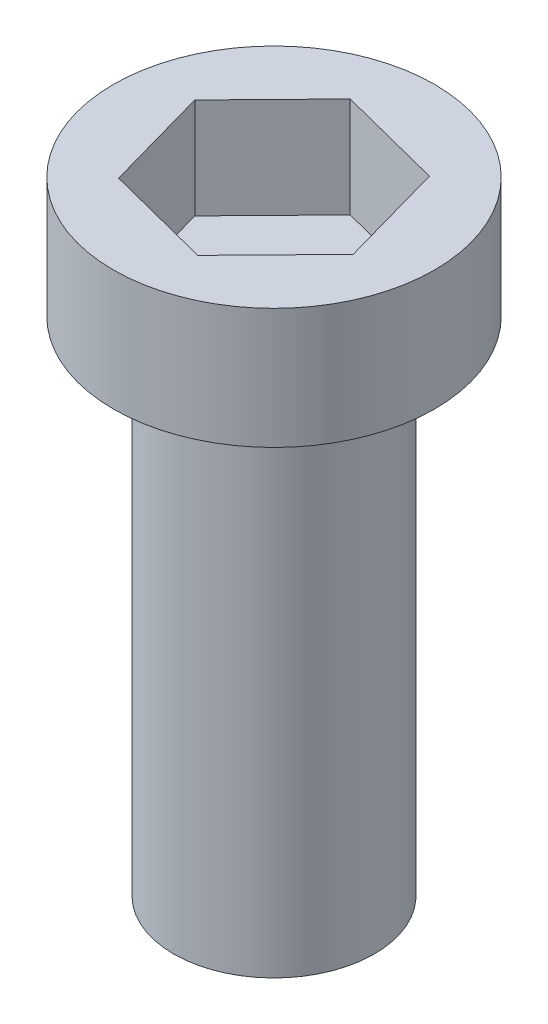
SolidWorks part; units mm, degrees
ref_plane "Front Plane" through (0, 0, 0) normal (0, 0, 1) x (1, 0, 0)
ref_plane "Top Plane" through (0, 0, 0) normal (0, 1, 0) x (1, 0, 0)
ref_plane "Right Plane" through (0, 0, 0) normal (1, 0, 0) x (0, 0, -1)
sketch "Sketch1" plane through (0, 0, 0) normal (0, 1, 0) x (1, 0, 0)
  circle A0 centre (0, 0) radius 5
  dimension "D1" = 10
extrude "Boss-Extrude1" add sketch "Sketch1" along normal blind 25
sketch "Sketch2" plane through (0, 25, 0) normal (0, 1, 0) x (1, 0, 0)
  circle A0 centre (0, 0) radius 8
  dimension "D1" = 16
extrude "Boss-Extrude2" add sketch "Sketch2" along normal blind 6
sketch "Sketch3" plane through (0, 31, 0) normal (0, 1, 0) x (1, 0, 0)
  line L1 (-1.475, 5.2698) -> (-5.3013, 1.3576)
  line L2 (-5.3013, 1.3576) -> (-3.8263, -3.9123)
  line L3 (-3.8263, -3.9123) -> (1.475, -5.2698)
  line L4 (1.475, -5.2698) -> (5.3013, -1.3576)
  line L5 (5.3013, -1.3576) -> (3.8263, 3.9123)
  line L6 (3.8263, 3.9123) -> (-1.475, 5.2698)
  circle A0 centre (0, 0) radius 4.7392 construction
extrude "Cut-Extrude1" cut sketch "Sketch3" against normal blind 5
